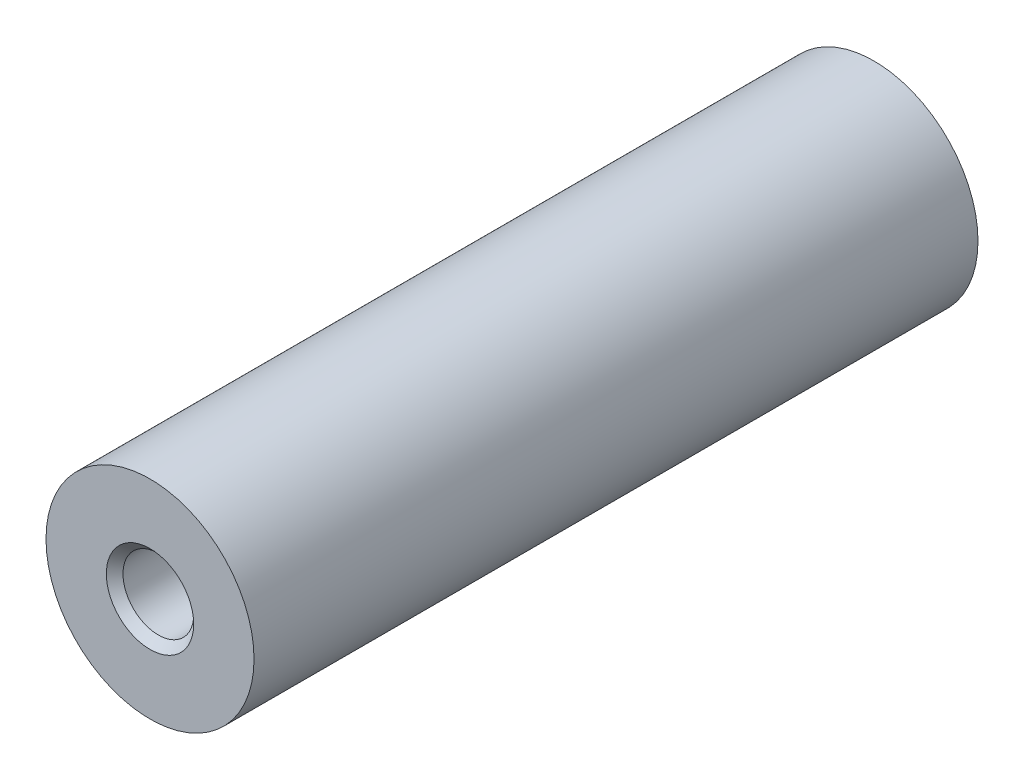
SolidWorks part; units mm, degrees
ref_plane "Front Plane" through (0, 0, 0) normal (0, 0, 1) x (1, 0, 0)
ref_plane "Top Plane" through (0, 0, 0) normal (0, 1, 0) x (1, 0, 0)
ref_plane "Right Plane" through (0, 0, 0) normal (1, 0, 0) x (0, 0, -1)
sketch "Sketch1" plane through (0, 0, 0) normal (0, 0, 1) x (1, 0, 0)
  circle A0 centre (0, 0) radius 12.5
extrude "Boss-Extrude1" add sketch "Sketch1" along normal blind 87
sketch "Sketch2" plane through (0, 0, 87) normal (0, 0, 1) x (1, 0, 0)
  circle A0 centre (0, 0) radius 4.25
extrude "Cut-Extrude1" cut sketch "Sketch2" against normal blind 25
sketch "Sketch3" plane through (0, 0, 87) normal (0, 0, 1) x (1, 0, 0)
  circle A0 centre (0, 0) radius 5
curve "Helix/Spiral1" pitch 1.5 height 15 turns 10
chamfer "Chamfer1" distance 1 angle 45 1 edges at (4.25, 0, 87)
